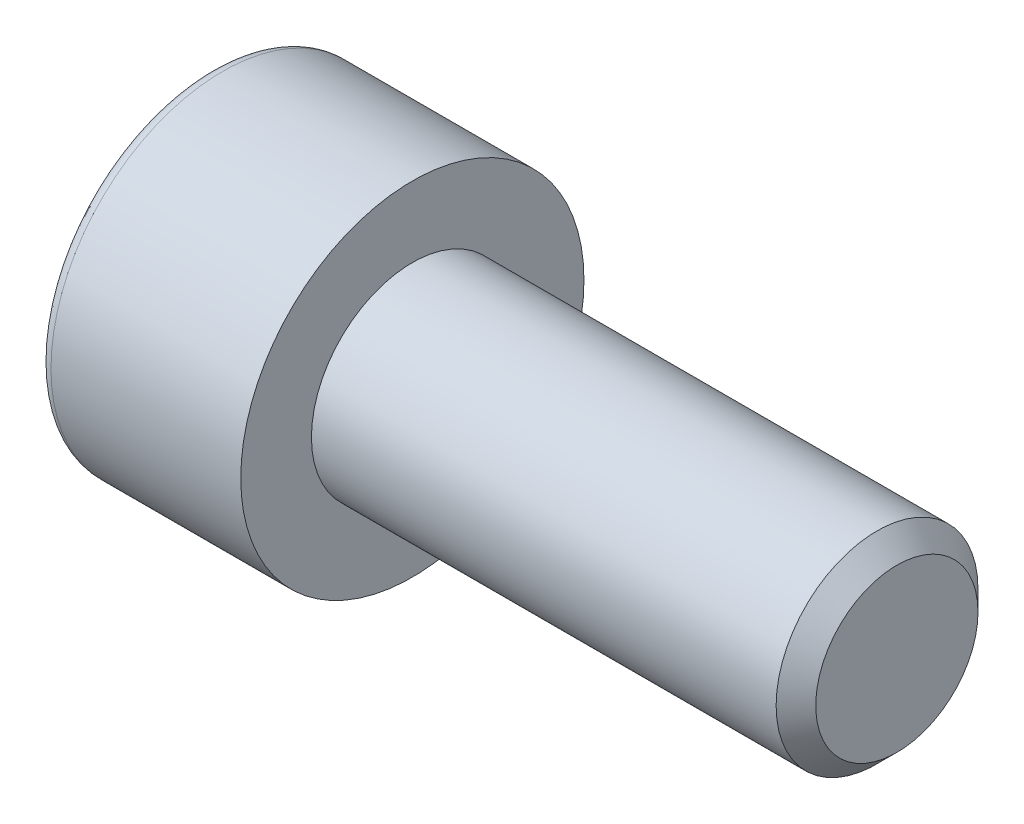
from build123d import *

# Parameters (mm, degrees)
CUT_EXTRUDE_1_DEPTH = 2.5


with BuildPart() as part:
    # 草图1 → 旋转1 (revolve)
    with BuildSketch(Plane.XY, mode=Mode.PRIVATE) as revolve_1_sk:
        with BuildLine():
            Line((17, 0), (17, -2.0095))
            Line((17, -2.0095), (16.5095, -2.5))
            Line((16.5095, -2.5), (5, -2.5))
            Line((5, -2.5), (5, -4.25))
            Line((5, -4.25), (0.3, -4.25))
            ThreePointArc((0.3, -4.25), (0.087867966, -4.162132034), (0, -3.95))
            Line((0, -3.95), (0, 0))
            Line((0, 0), (17, 0))
        make_face()
    revolve(revolve_1_sk.sketch.rotate(Axis((0, 0, 0), (1, 0, 0)), 90), axis=Axis((0, 0, 0), (1, 0, 0)))

    # 草图2 → 切除-拉伸1 (cut)
    with BuildSketch(Plane(origin=(0, 0, 0), x_dir=(0, 0, -1), z_dir=(1, 0, 0))):
        Polygon((-1.7, -0.981495458), (0, -1.962990915), (1.7, -0.981495458), (1.7, 0.981495458), (0, 1.962990915), (-1.7, 0.981495458), align=None)
    extrude(amount=CUT_EXTRUDE_1_DEPTH, mode=Mode.SUBTRACT)


solid = part.part
